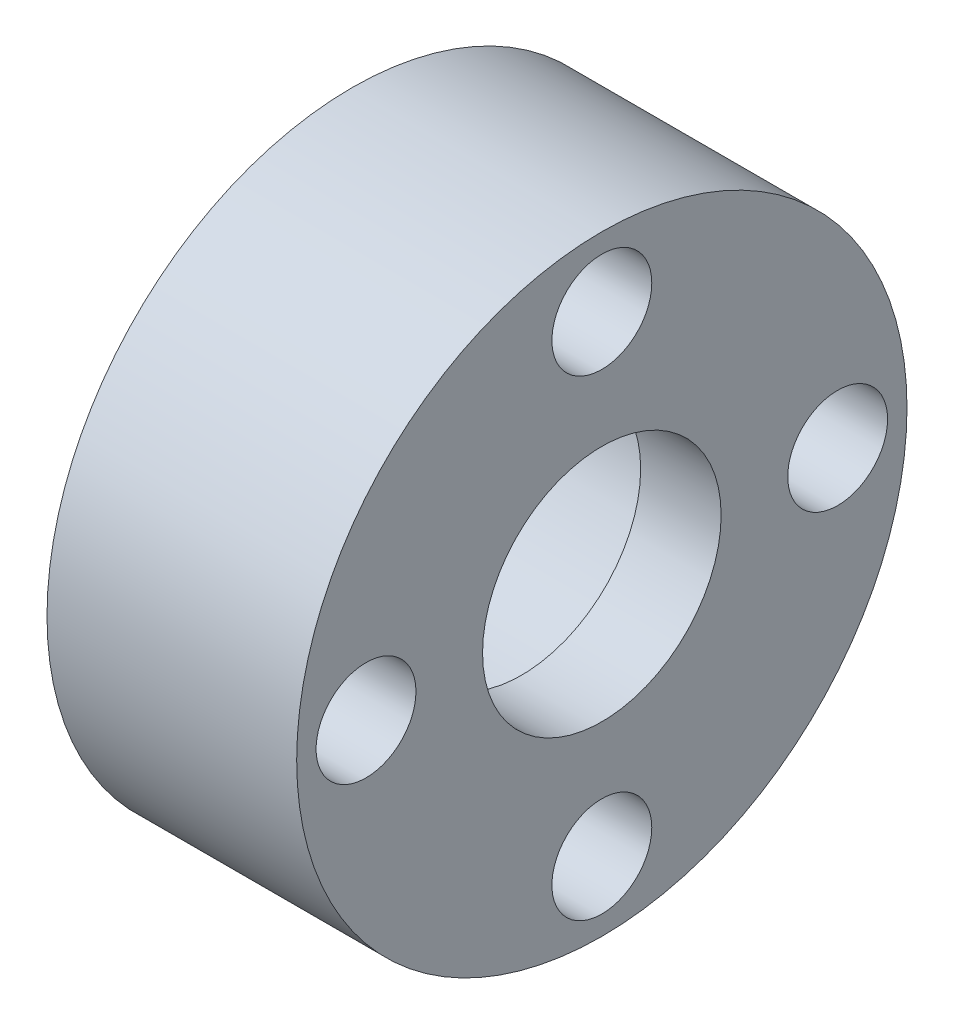
from build123d import *

# Parameters (mm, degrees)
HOLE_SIZE_PER_SOCKET_HEAD_CAP_SCREW_TYPE_D           = 11
HOLE_SIZE_PER_SOCKET_HEAD_CAP_SCREW_TYPE_CBORE_D     = 18
HOLE_SIZE_PER_SOCKET_HEAD_CAP_SCREW_TYPE_CBORE_DEPTH = 20


with BuildPart() as part:
    # Sketch1 → Revolve1 (revolve)
    with BuildSketch(Plane.XY, mode=Mode.PRIVATE) as revolve1_sk:
        Polygon((48.914797255, 21.5), (63.414797255, 21.5), (63.414797255, 55), (18.414797255, 55), (18.414797255, 30), (48.914797255, 30), align=None)
    revolve(revolve1_sk.sketch.rotate(Axis((0, 0, 0), (1, 0, 0)), 90), axis=Axis((0, 0, 0), (1, 0, 0)))

    # Hole size per socket head cap screw type1 (through all)
    with Locations(Plane(origin=(63.414797255, 0, 0), x_dir=(0, 0, -1), z_dir=(1, 0, 0))):
        with Locations((0, 42.5), (0, -42.5), (-42.5, 0), (42.5, 0)):
            CounterBoreHole(HOLE_SIZE_PER_SOCKET_HEAD_CAP_SCREW_TYPE_D / 2, HOLE_SIZE_PER_SOCKET_HEAD_CAP_SCREW_TYPE_CBORE_D / 2, HOLE_SIZE_PER_SOCKET_HEAD_CAP_SCREW_TYPE_CBORE_DEPTH)


solid = part.part
